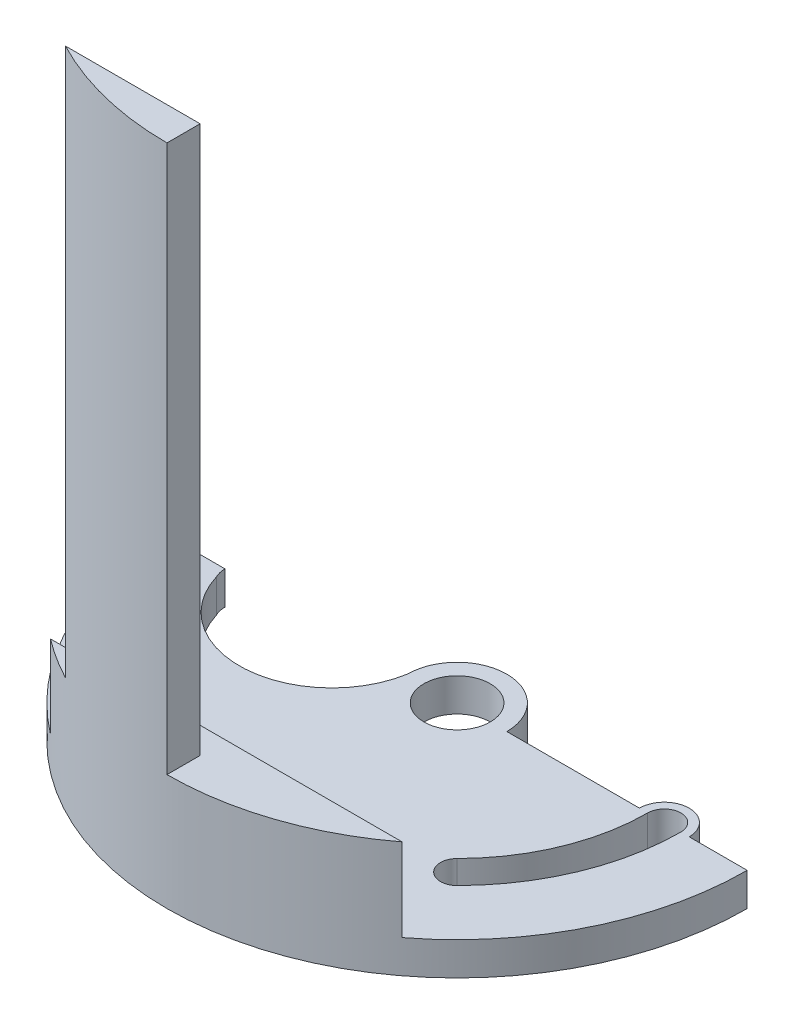
SolidWorks part; units mm, degrees
ref_plane "Front Plane" through (0, 0, 0) normal (0, 0, 1) x (1, 0, 0)
ref_plane "Top Plane" through (0, 0, 0) normal (0, 1, 0) x (1, 0, 0)
ref_plane "Right Plane" through (0, 0, 0) normal (1, 0, 0) x (0, 0, -1)
other "Configuration Table"
sketch "Sketch1" plane through (0, 0, 0) normal (0, 1, 0) x (1, 0, 0)
  circle A0 centre (0, 0) radius 17.5
  dimension "D1" = 35
extrude "Boss-Extrude1" add sketch "Sketch1" along normal blind 30
sketch "Sketch2" plane through (0, 0, 0) normal (0, -1, 0) x (1, 0, 0)
  circle A0 centre (0, 0) radius 4
  dimension "D1" = 8
extrude "Boss-Extrude2" add sketch "Sketch2" along normal blind 2
chamfer "Chamfer1" distance 1 angle 45 1 edges at (0, 0, -4)
sketch "Sketch4" plane through (0, -2, 0) normal (0, -1, 0) x (1, 0, 0)
  circle A0 centre (0, 0) radius 2
  dimension "D1" = 4
extrude "Boss-Extrude3" add sketch "Sketch4" along normal blind 12
sketch "Sketch5" plane through (0, -14, 0) normal (0, -1, 0) x (1, 0, 0)
  circle A0 centre (0, 0) radius 1.5
  dimension "D1" = 3
extrude "Cut-Extrude1" cut sketch "Sketch5" against normal blind 12
sketch "Sketch6" plane through (0, 0, 0) normal (1, 0, 0) x (0, 0, -1)
  line L0 (0, 30) -> (0, -49970) construction
  line L1 (17.5, 30) -> (-17.5, 30) construction
  line L2 (-17.5, 0) -> (17.5, 0) construction
  line L3 (-12.5, 30) -> (21.7943, 30)
  line L4 (-12.5, 30) -> (-12.5, 2)
  line L5 (-12.5, 2) -> (21.7943, 2)
  line L6 (21.7943, 30) -> (21.7943, 2)
  line L7 (-17.5, 30) -> (-17.5, 0) construction
  point P4 (0, 30)
  dimension "D1" = 2
  dimension "D2" = 5
extrude "Cut-Extrude2" cut sketch "Sketch6" against normal through all both and the other way through all
sketch "Sketch7" plane through (0, 0, 0) normal (1, 0, 0) x (0, 0, -1)
  line L0 (-17.5, 0) -> (17.5, 0) construction
  line L1 (-12.5, 30) -> (-15.5, 30)
  line L2 (-12.5, 30) -> (-12.5, 7)
  line L3 (-12.5, 7) -> (-15.5, 7)
  line L4 (-15.5, 30) -> (-15.5, 7)
  dimension "D1" = 7
  dimension "D2" = 3
extrude "Cut-Extrude3" cut sketch "Sketch7" against normal through all both and the other way through all
sketch "Sketch8" plane through (0, 0, 0) normal (1, 0, 0) x (0, 0, -1)
  line L0 (-12.5, 2) -> (-50012.5, 2) construction
  line L2 (-12.5, 7) -> (-14, 7)
  line L3 (-12.5, 7) -> (-12.5, 2)
  line L4 (-12.5, 2) -> (-14, 2)
  line L5 (-14, 7) -> (-14, 2)
  dimension "D1" = 1.5
extrude "Cut-Extrude4" cut sketch "Sketch8" against normal through all both and the other way through all
sketch "Sketch9" plane through (0, 0, 15.5) normal (0, 0, -1) x (-1, 0, 0)
  line L0 (-10.5, 7) -> (10.5, 7) construction
  line L1 (-8.124, 30) -> (0, 30)
  line L2 (-8.124, 30) -> (-8.124, 7)
  line L3 (-8.124, 7) -> (0, 7)
  line L4 (0, 30) -> (0, 7)
extrude "Cut-Extrude5" cut sketch "Sketch9" against normal through all both and the other way through all
sketch "Sketch10" plane through (0, 30, 0) normal (0, 1, 0) x (1, 0, 0)
  circle A0 centre (-1.034, -16.5233) radius 0.6413
extrude "Cut-Extrude6" cut sketch "Sketch10" against normal blind 0.5 and the other way through all
sketch "Sketch11" plane through (0, 2, 0) normal (0, 1, 0) x (1, 0, 0)
  circle A0 centre (0, 0) radius 17.5
extrude "Boss-Extrude4" add sketch "Sketch11" along normal up to surface (5 mm away) up to face at (-1.574, 7, 15.4799)
sketch "Sketch12" plane through (0, 7, 0) normal (0, 1, 0) x (1, 0, 0)
  line L0 (0, 0) -> (0, -50000) construction
  line L1 (0, 0) -> (-50000, 0) construction
  line L2 (-17.5, 0) -> (-3, 0)
  line L3 (3, 0) -> (11, 0)
  line L4 (14, 0) -> (18.5714, 0)
  line L5 (-17.5, 0) -> (-17.5, 21.355)
  line L6 (-17.5, 21.355) -> (18.5714, 21.355)
  line L7 (18.5714, 21.355) -> (18.5714, 0)
  circle A0 centre (0, 0) radius 12.5 construction
  arc A2 (14, 0) -> (11, 0) centre (12.5, 0) ccw
  arc A3 (3, 0) -> (-3, 0) centre (0, 0) ccw
  circle A4 centre (0, 0) radius 17.5 construction
  dimension "D1" = 25
  dimension "D2" = 3
  dimension "D4" = 6
extrude "Cut-Extrude8" cut sketch "Sketch12" against normal blind 4
sketch "Sketch13" plane through (0, 0, 0) normal (1, 0, 0) x (0, 0, -1)
  line L0 (0, 7) -> (-17.5, 7) construction
  line L1 (-13.9225, 7) -> (5.3458, 7)
  line L2 (-13.9225, 7) -> (-13.9225, 5)
  line L3 (-13.9225, 5) -> (5.3458, 5)
  line L4 (5.3458, 7) -> (5.3458, 5)
extrude "Cut-Extrude9" cut sketch "Sketch13" against normal through all both and the other way through all
sketch "Sketch14" plane through (0, 5, 0) normal (0, 1, 0) x (1, 0, 0)
  circle A0 centre (0, 0) radius 2
  dimension "D1" = 4
extrude "Cut-Extrude10" cut sketch "Sketch14" against normal blind 6
sketch "Sketch16" plane through (0, 0, 0) normal (1, 0, 0) x (0, 0, -1)
  line L0 (-17.5, 0) -> (17.5, 0) construction
  line L1 (17.5, 3) -> (14.25, 3)
  line L2 (17.5, 3) -> (17.5, 0)
  line L3 (17.5, 0) -> (14.25, 0)
  line L4 (14.25, 3) -> (14.25, 0)
  dimension "D1" = 3.25
extrude "Cut-Extrude11" cut sketch "Sketch16" against normal through all both and the other way through all
sketch "Sketch17" plane through (0, 5, 0) normal (0, 1, 0) x (1, 0, 0)
  line L0 (0, 0) -> (35355.3391, -35355.3391) construction
  line L1 (0, 0) -> (50000, 0) construction
  circle A0 centre (0, 0) radius 12.5 construction
  arc A1 (12.5, 0) -> (8.8388, -8.8388) centre (0, 0) cw construction
  arc A2 (9.5459, -9.5459) -> (13.5, 0) centre (0, 0) ccw
  arc A3 (8.1317, -8.1317) -> (11.5, 0) centre (0, 0) ccw
  arc A4 (8.1317, -8.1317) -> (9.5459, -9.5459) centre (8.8388, -8.8388) ccw
  arc A5 (13.5, 0) -> (11.5, 0) centre (12.5, 0) ccw
  point P6 (11.5485, -4.7835)
  dimension "D1" = 1
  dimension "D2" = 45
extrude "Cut-Extrude12" cut sketch "Sketch17" against normal through all
sketch "Sketch18" plane through (0, 3, 0) normal (0, 1, 0) x (1, 0, 0)
  circle A0 centre (0, 0) radius 17.5
  dimension "D1" = 35
extrude "Cut-Extrude13" cut sketch "Sketch18" against normal up to surface (17 mm away) up to face at (0, -14, -1.5)
sketch "Sketch19" plane through (0, 7, 0) normal (0, 1, 0) x (1, 0, 0)
  line L3 (10.6026, -13.9225) -> (-10.6026, -13.9225)
  line L4 (-8.124, -15.5) -> (0, -15.5)
  line L5 (0, -15.5) -> (0, -17.5)
  line L6 (10.6026, -13.9225) -> (-10.6026, -13.9225)
  line L7 (-8.124, -15.5) -> (0, -15.5)
  line L8 (0, -15.5) -> (0, -17.5)
  arc A2 (0, -17.5) -> (10.6026, -13.9225) centre (0, 0) ccw
  arc A3 (-10.6026, -13.9225) -> (-8.124, -15.5) centre (0, 0) ccw
  arc A4 (0, -17.5) -> (10.6026, -13.9225) centre (0, 0) ccw
  arc A5 (-10.6026, -13.9225) -> (-8.124, -15.5) centre (0, 0) ccw
  dimension "D1" = 0
extrude "Boss-Extrude5" add sketch "Sketch19" along normal blind 3
sketch "Sketch20" plane through (0, 30, 0) normal (0, 1, 0) x (1, 0, 0)
  line L2 (0, -17.5) -> (0, -15.5)
  line L3 (0, -15.5) -> (-8.124, -15.5)
  line L4 (0, -17.5) -> (0, -15.5)
  line L5 (0, -15.5) -> (-8.124, -15.5)
  arc A1 (-8.124, -15.5) -> (0, -17.5) centre (0, 0) ccw
  arc A2 (-8.124, -15.5) -> (0, -17.5) centre (0, 0) ccw
  dimension "D1" = 0
extrude "Boss-Extrude6" add sketch "Sketch20" along normal blind 13
sketch "Sketch21" plane through (0, 5, 0) normal (0, 1, 0) x (1, 0, 0)
  circle A0 centre (0, 0) radius 12.5 construction
  circle A1 centre (-12.5, 0) radius 1.5
  dimension "D1" = 3
extrude "Cut-Extrude14" cut sketch "Sketch21" against normal through all both and the other way through all
sketch "Sketch22" plane through (0, 5, 0) normal (0, 1, 0) x (1, 0, 0)
  circle A0 centre (0, 0) radius 12.5 construction
  circle A1 centre (-10.5808, -6.6555) radius 1
  dimension "D1" = 2
extrude "Boss-Extrude7" add sketch "Sketch22" along normal blind 5
sketch "Sketch23" plane through (0, 5, 0) normal (0, 1, 0) x (1, 0, 0)
  line L0 (-14, 0) -> (-3, 0)
  arc A0 (-14, 0) -> (-3, 0) centre (-8.5, 0.9449) ccw
extrude "Cut-Extrude15" cut sketch "Sketch23" against normal blind 5
